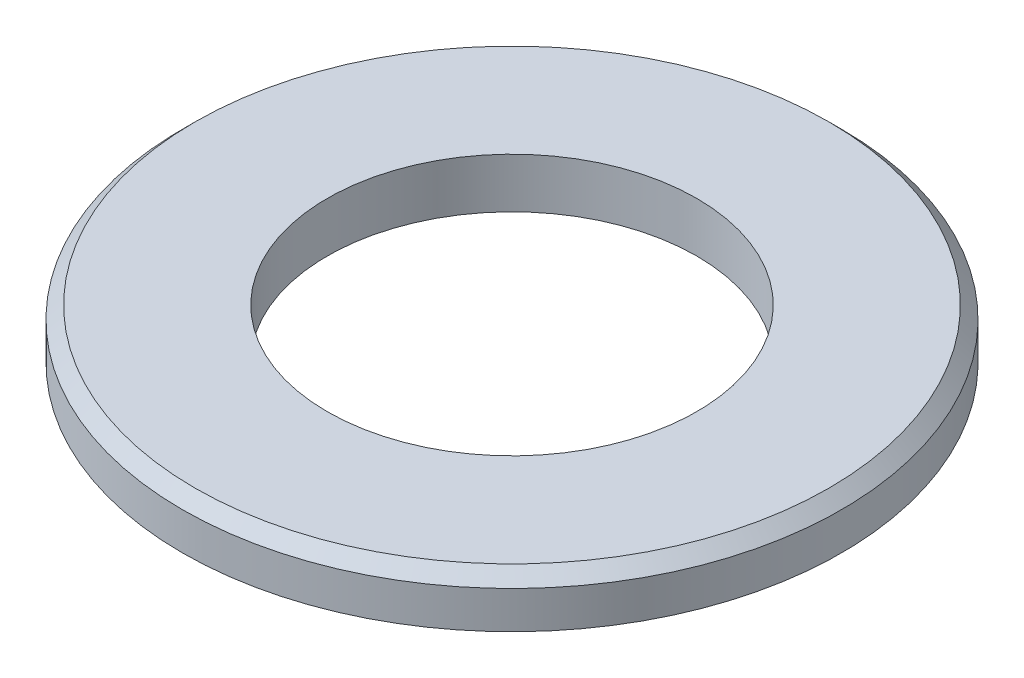
from build123d import *


with BuildPart() as part:
    # 草图1 → Revolve 481 (revolve)
    with BuildSketch(Plane.XY, mode=Mode.PRIVATE) as revolve_481_sk:
        Polygon((-31.75, 13.644507042), (-33, 12.394507042), (-33, 8.644507042), (-18.5, 8.644507042), (-18.5, 13.644507042), align=None)
    revolve(revolve_481_sk.sketch.rotate(Axis((0, 0, 0), (0, 1, 0)), 270), axis=Axis((0, 0, 0), (0, 1, 0)))


solid = part.part
